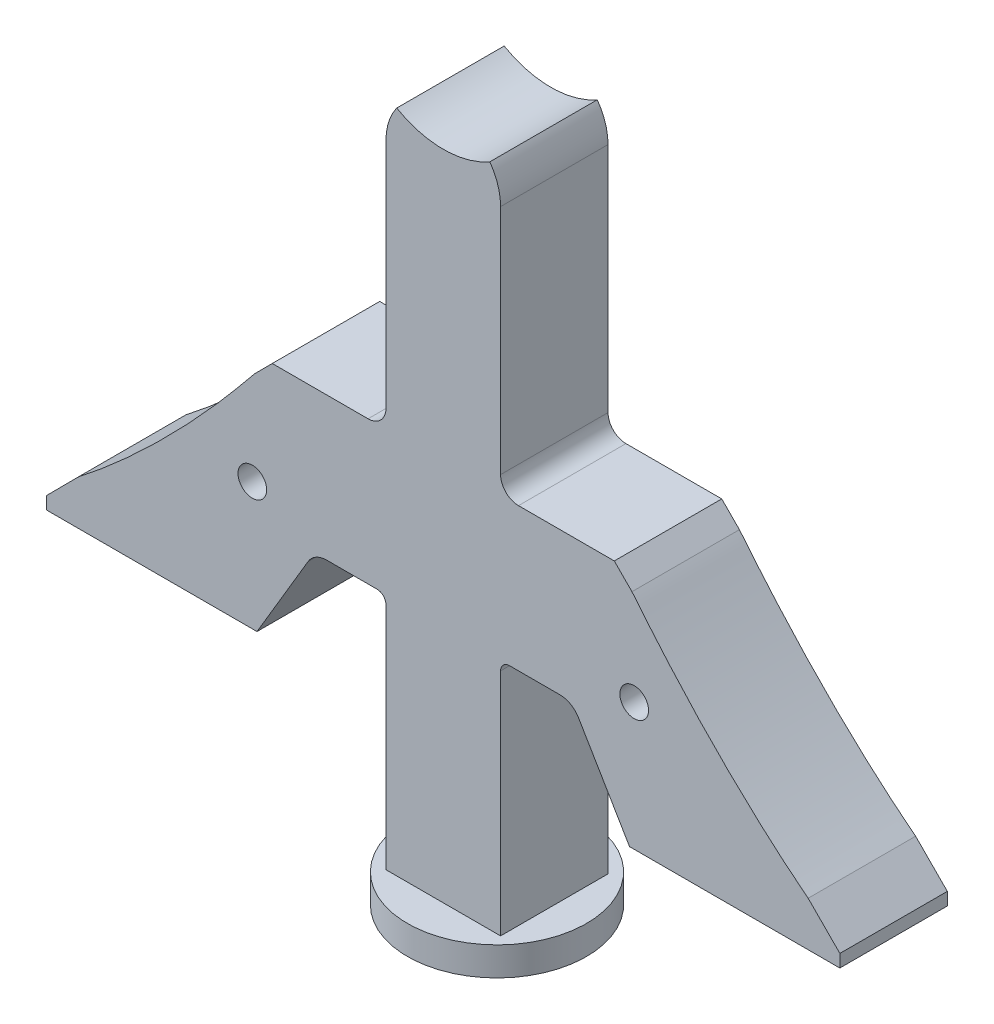
SolidWorks part; units mm, degrees
ref_plane "Front Plane" through (0, 0, 0) normal (0, 0, 1) x (1, 0, 0)
ref_plane "Top Plane" through (0, 0, 0) normal (0, 1, 0) x (1, 0, 0)
ref_plane "Right Plane" through (0, 0, 0) normal (1, 0, 0) x (0, 0, -1)
sketch "Sketch1" plane through (0, 0, 0) normal (0, 0, 1) x (1, 0, 0)
  line L0 (-15, 37.0303) -> (-15, -127.658)
  line L1 (15, 37.0303) -> (15, -127.658)
  line L2 (-15, -127.658) -> (15, -127.658)
  arc A3 (15, 37.0303) -> (-15, 37.0303) centre (0, 37.0303) ccw
extrude "Boss-Extrude1" add sketch "Sketch1" along normal blind 10
sketch "Sketch2" plane through (0, 0, 0) normal (0, 0, -1) x (-1, 0, 0)
  line L25 (0, -15) -> (30.09, -15)
  line L29 (139.2471, -124.8835) -> (-139.2471, -124.8835)
  line L30 (0, 159.5195) -> (0, -140.4805) construction
  line L31 (0, -15) -> (-30.09, -15)
  line L32 (30.09, -15) -> (139.2471, -124.8835)
  line L34 (-30.09, -15) -> (-139.2471, -124.8835)
  dimension "D1" = 45.19
  dimension "D2" = 45.19
  dimension "D3" = 30.09
  dimension "D4" = 30.09
extrude "Boss-Extrude2" add sketch "Sketch2" against normal blind 10
sketch "Sketch72" plane through (0, 0, 10) normal (0, 0, 1) x (1, 0, 0)
  circle A0 centre (0, 37.0303) radius 5
extrude "Cut-Extrude2" cut sketch "Sketch72" against normal blind 10
sketch "Sketch75" plane through (0, 0, 10) normal (0, 0, 1) x (1, 0, 0)
  line L2 (-101.3658, -86.7501) -> (-101.3003, -86.8152)
sketch "Sketch76" plane through (0, 0, 10) normal (0, 0, 1) x (1, 0, 0)
  line L2 (-100.6847, -86.0644) -> (-100.5316, -86.2165)
sketch "Sketch77" plane through (0, 0, 10) normal (0, 0, 1) x (1, 0, 0)
  line L2 (-99.9976, -85.3728) -> (-99.7607, -85.6082)
sketch "Sketch78" plane through (0, 0, 10) normal (0, 0, 1) x (1, 0, 0)
  circle A0 centre (-65.1228, -29.2131) radius 15
sketch "Sketch79" plane through (0, 0, 10) normal (0, 0, 1) x (1, 0, 0)
  circle A0 centre (-63.7391, -27.6067) radius 15
sketch "Sketch80" plane through (0, 0, 10) normal (0, 0, 1) x (1, 0, 0)
  line L2 (-99.3047, -84.6753) -> (-98.9873, -84.9906)
sketch "Sketch81" plane through (0, 0, 10) normal (0, 0, 1) x (1, 0, 0)
  line L2 (-98.6059, -83.9719) -> (-98.2113, -84.3638)
sketch "Sketch82" plane through (0, 0, 10) normal (0, 0, 1) x (1, 0, 0)
  line L2 (-97.9012, -83.2624) -> (-97.4325, -83.728)
sketch "Sketch83" plane through (0, 0, 10) normal (0, 0, 1) x (1, 0, 0)
  line L2 (-97.1906, -82.5471) -> (-96.6508, -83.0833)
sketch "Sketch84" plane through (0, 0, 10) normal (0, 0, 1) x (1, 0, 0)
  line L2 (-96.474, -81.8257) -> (-95.866, -82.4297)
sketch "Sketch85" plane through (0, 0, 10) normal (0, 0, 1) x (1, 0, 0)
  line L2 (-95.7514, -81.0984) -> (-95.078, -81.7673)
sketch "Sketch86" plane through (0, 0, 10) normal (0, 0, 1) x (1, 0, 0)
  line L2 (-95.0229, -80.365) -> (-94.2869, -81.0962)
sketch "Sketch88" plane through (0, 0, 10) normal (0, 0, 1) x (1, 0, 0)
  line L2 (-94.2885, -79.6257) -> (-93.4926, -80.4163)
sketch "Sketch89" plane through (0, 0, 10) normal (0, 0, 1) x (1, 0, 0)
  line L2 (-92.8017, -78.129) -> (-91.8942, -79.0305)
sketch "Sketch90" plane through (0, 0, 10) normal (0, 0, 1) x (1, 0, 0)
  line L1 (-93.5481, -78.8804) -> (-92.695, -79.7278)
sketch "Sketch91" plane through (0, 0, 10) normal (0, 0, 1) x (1, 0, 0)
  line L2 (-92.0494, -77.3717) -> (-91.0901, -78.3246)
sketch "Sketch92" plane through (0, 0, 10) normal (0, 0, 1) x (1, 0, 0)
  line L2 (-91.2911, -76.6083) -> (-90.2828, -77.61)
sketch "Sketch94" plane through (0, 0, 10) normal (0, 0, 1) x (1, 0, 0)
  line L2 (-89.7566, -75.0637) -> (-88.6584, -76.1546)
sketch "Sketch95" plane through (0, 0, 10) normal (0, 0, 1) x (1, 0, 0)
  line L2 (-90.5268, -75.839) -> (-89.4722, -76.8866)
sketch "Sketch96" plane through (0, 0, 10) normal (0, 0, 1) x (1, 0, 0)
  line L2 (-88.9805, -74.2823) -> (-87.8414, -75.4138)
sketch "Sketch97" plane through (0, 0, 10) normal (0, 0, 1) x (1, 0, 0)
  line L2 (-88.1983, -73.495) -> (-87.0213, -74.6643)
sketch "Sketch98" plane through (0, 0, 10) normal (0, 0, 1) x (1, 0, 0)
  line L2 (-87.4103, -72.7017) -> (-86.198, -73.906)
sketch "Sketch99" plane through (0, 0, 10) normal (0, 0, 1) x (1, 0, 0)
  line L2 (-86.6163, -71.9024) -> (-85.3716, -73.1388)
sketch "Sketch100" plane through (0, 0, 10) normal (0, 0, 1) x (1, 0, 0)
  line L2 (-85.8163, -71.0971) -> (-84.5422, -72.3629)
sketch "Sketch101" plane through (0, 0, 10) normal (0, 0, 1) x (1, 0, 0)
  line L2 (-85.0104, -70.2859) -> (-83.7097, -71.578)
sketch "Sketch102" plane through (0, 0, 10) normal (0, 0, 1) x (1, 0, 0)
  line L2 (-84.1986, -69.4686) -> (-82.8742, -70.7842)
sketch "Sketch103" plane through (0, 0, 10) normal (0, 0, 1) x (1, 0, 0)
  line L2 (-82.5572, -67.8163) -> (-81.1946, -69.1699)
sketch "Sketch104" plane through (0, 0, 10) normal (0, 0, 1) x (1, 0, 0)
  line L2 (-83.3808, -68.6454) -> (-82.0358, -69.9815)
sketch "Sketch105" plane through (0, 0, 10) normal (0, 0, 1) x (1, 0, 0)
  line L2 (-81.7276, -66.9812) -> (-80.3504, -68.3492)
sketch "Sketch106" plane through (0, 0, 10) normal (0, 0, 1) x (1, 0, 0)
  line L2 (-80.892, -66.1401) -> (-79.5035, -67.5194)
sketch "Sketch107" plane through (0, 0, 10) normal (0, 0, 1) x (1, 0, 0)
  line L2 (-80.0506, -65.2931) -> (-78.6539, -66.6806)
sketch "Sketch108" plane through (0, 0, 0) normal (0, 0, 1) x (1, 0, 0)
  line L2 (-79.2033, -64.4401) -> (-77.8016, -65.8326)
sketch "Sketch109" plane through (0, 0, 0) normal (0, 0, 1) x (1, 0, 0)
  line L2 (-78.3501, -63.5812) -> (-76.9466, -64.9754)
sketch "Sketch110" plane through (0, 0, 10) normal (0, 0, 1) x (1, 0, 0)
  line L2 (-77.4909, -62.7164) -> (-76.0891, -64.109)
sketch "Sketch111" plane through (0, 0, 10) normal (0, 0, 1) x (1, 0, 0)
  line L2 (-75.7551, -60.9689) -> (-74.3666, -62.3482)
sketch "Sketch112" plane through (0, 0, 10) normal (0, 0, 1) x (1, 0, 0)
  line L1 (-76.6259, -61.8456) -> (-75.2291, -63.2333)
sketch "Sketch113" plane through (0, 0, 10) normal (0, 0, 1) x (1, 0, 0)
  line L2 (-74.8783, -60.0863) -> (-73.5017, -61.4539)
sketch "Sketch115" plane through (0, 0, 10) normal (0, 0, 1) x (1, 0, 0)
  line L2 (-73.9957, -59.1978) -> (-72.6344, -60.5501)
sketch "Sketch116" plane through (0, 0, 10) normal (0, 0, 1) x (1, 0, 0)
  line L2 (-73.1072, -58.3034) -> (-71.7649, -59.6368)
sketch "Sketch117" plane through (0, 0, 10) normal (0, 0, 1) x (1, 0, 0)
  line L2 (-72.2128, -57.4031) -> (-70.8932, -58.714)
sketch "Sketch118" plane through (0, 0, 10) normal (0, 0, 1) x (1, 0, 0)
  line L2 (-71.3126, -56.4969) -> (-70.0193, -57.7817)
sketch "Sketch119" plane through (0, 0, 10) normal (0, 0, 1) x (1, 0, 0)
  line L2 (-70.4066, -55.5848) -> (-69.1433, -56.8397)
sketch "Sketch120" plane through (0, 0, 10) normal (0, 0, 1) x (1, 0, 0)
  line L2 (-69.4947, -54.6669) -> (-68.2654, -55.8881)
sketch "Sketch121" plane through (0, 0, 10) normal (0, 0, 1) x (1, 0, 0)
  line L2 (-68.577, -53.7431) -> (-67.3854, -54.9268)
sketch "Sketch122" plane through (0, 0, 10) normal (0, 0, 1) x (1, 0, 0)
  line L2 (-67.6534, -52.8134) -> (-66.5036, -53.9556)
sketch "Sketch123" plane through (0, 0, 10) normal (0, 0, 1) x (1, 0, 0)
  line L2 (-66.7241, -51.8778) -> (-65.6199, -52.9747)
sketch "Sketch124" plane through (0, 0, 10) normal (0, 0, 1) x (1, 0, 0)
  line L2 (-65.7889, -50.9365) -> (-64.7345, -51.9839)
sketch "Sketch125" plane through (0, 0, 10) normal (0, 0, 1) x (1, 0, 0)
  line L2 (-64.8479, -49.9892) -> (-63.8474, -50.9831)
sketch "Sketch126" plane through (0, 0, 10) normal (0, 0, 1) x (1, 0, 0)
  line L2 (-63.9012, -49.0361) -> (-62.9587, -49.9724)
sketch "Sketch127" plane through (0, 0, 10) normal (0, 0, 1) x (1, 0, 0)
  line L2 (-62.9486, -48.0772) -> (-62.0684, -48.9516)
sketch "Sketch128" plane through (0, 0, 10) normal (0, 0, 1) x (1, 0, 0)
  line L2 (-61.9903, -47.1125) -> (-61.1767, -47.9207)
sketch "Sketch129" plane through (0, 0, 10) normal (0, 0, 1) x (1, 0, 0)
  line L2 (-61.0261, -46.142) -> (-60.2836, -46.8796)
sketch "Sketch130" plane through (0, 0, 10) normal (0, 0, 1) x (1, 0, 0)
  line L2 (-60.0562, -45.1657) -> (-59.3892, -45.8283)
sketch "Sketch131" plane through (0, 0, 10) normal (0, 0, 1) x (1, 0, 0)
  line L2 (-59.0806, -44.1835) -> (-58.4935, -44.7668)
sketch "Sketch132" plane through (0, 0, 10) normal (0, 0, 1) x (1, 0, 0)
  line L2 (-58.0992, -43.1956) -> (-57.5966, -43.6949)
sketch "Sketch133" plane through (0, 0, 10) normal (0, 0, 1) x (1, 0, 0)
  line L2 (-57.1121, -42.2019) -> (-56.6986, -42.6126)
sketch "Sketch134" plane through (0, 0, 10) normal (0, 0, 1) x (1, 0, 0)
  line L2 (-56.1192, -41.2024) -> (-55.7997, -41.5198)
sketch "Sketch135" plane through (0, 0, 10) normal (0, 0, 1) x (1, 0, 0)
  line L2 (-55.1206, -40.1971) -> (-54.8997, -40.4165)
sketch "Sketch136" plane through (0, 0, 10) normal (0, 0, 1) x (1, 0, 0)
  line L2 (-54.1162, -39.1861) -> (-53.999, -39.3026)
sketch "Sketch137" plane through (0, 0, 10) normal (0, 0, 1) x (1, 0, 0)
  line L0 (-101.3003, -86.8152) -> (-100.5316, -86.2165)
  line L1 (-100.5316, -86.2165) -> (-99.7607, -85.6082)
  line L2 (-99.7607, -85.6082) -> (-98.9873, -84.9906)
  line L3 (-98.9873, -84.9906) -> (-98.2113, -84.3638)
  line L4 (-98.2113, -84.3638) -> (-97.4325, -83.728)
  line L5 (-97.4325, -83.728) -> (-96.6508, -83.0833)
  line L6 (-96.6508, -83.0833) -> (-95.866, -82.4297)
  line L7 (-95.866, -82.4297) -> (-95.078, -81.7673)
  line L8 (-95.078, -81.7673) -> (-94.2869, -81.0962)
  line L9 (-94.2869, -81.0962) -> (-93.4926, -80.4163)
  line L10 (-93.4926, -80.4163) -> (-92.695, -79.7278)
  line L11 (-92.695, -79.7278) -> (-91.8942, -79.0305)
  line L12 (-91.8942, -79.0305) -> (-91.0901, -78.3246)
  line L13 (-91.0901, -78.3246) -> (-90.2828, -77.61)
  line L14 (-90.2828, -77.61) -> (-89.4722, -76.8866)
  line L15 (-89.4722, -76.8866) -> (-88.6584, -76.1546)
  line L16 (-88.6584, -76.1546) -> (-87.8414, -75.4138)
  line L17 (-87.8414, -75.4138) -> (-87.0213, -74.6643)
  line L18 (-87.0213, -74.6643) -> (-86.198, -73.906)
  line L19 (-86.198, -73.906) -> (-85.3716, -73.1388)
  line L20 (-85.3716, -73.1388) -> (-84.5422, -72.3629)
  line L21 (-84.5422, -72.3629) -> (-83.7097, -71.578)
  line L22 (-83.7097, -71.578) -> (-82.8742, -70.7842)
  line L23 (-82.8742, -70.7842) -> (-82.0358, -69.9815)
  line L24 (-82.0358, -69.9815) -> (-81.1946, -69.1699)
  line L25 (-81.1946, -69.1699) -> (-80.3504, -68.3492)
  line L26 (-80.3504, -68.3492) -> (-79.5035, -67.5194)
  line L27 (-79.5035, -67.5194) -> (-78.6539, -66.6806)
  line L28 (-78.6539, -66.6806) -> (-77.8016, -65.8326)
  line L29 (-77.8016, -65.8326) -> (-76.9466, -64.9754)
  line L30 (-76.9466, -64.9754) -> (-76.0891, -64.109)
  line L31 (-76.0891, -64.109) -> (-75.2291, -63.2333)
  line L32 (-75.2291, -63.2333) -> (-74.3666, -62.3482)
  line L33 (-74.3666, -62.3482) -> (-73.5017, -61.4539)
  line L34 (-73.5017, -61.4539) -> (-72.6344, -60.5501)
  line L35 (-72.6344, -60.5501) -> (-71.7649, -59.6368)
  line L36 (-71.7649, -59.6368) -> (-70.8932, -58.714)
  line L37 (-70.8932, -58.714) -> (-70.0193, -57.7817)
  line L38 (-70.0193, -57.7817) -> (-69.1433, -56.8397)
  line L39 (-69.1433, -56.8397) -> (-68.2654, -55.8881)
  line L40 (-68.2654, -55.8881) -> (-67.3854, -54.9268)
  line L41 (-67.3854, -54.9268) -> (-66.5036, -53.9556)
  line L42 (-66.5036, -53.9556) -> (-65.6199, -52.9747)
  line L43 (-65.6199, -52.9747) -> (-64.7345, -51.9839)
  line L44 (-64.7345, -51.9839) -> (-63.8474, -50.9831)
  line L45 (-63.8474, -50.9831) -> (-62.9587, -49.9724)
  line L46 (-62.9587, -49.9724) -> (-62.0684, -48.9516)
  line L47 (-62.0684, -48.9516) -> (-61.1767, -47.9207)
  line L48 (-61.1767, -47.9207) -> (-60.2836, -46.8796)
  line L49 (-60.2836, -46.8796) -> (-59.3892, -45.8283)
  line L50 (-59.3892, -45.8283) -> (-58.4935, -44.7668)
  line L51 (-58.4935, -44.7668) -> (-57.5966, -43.6949)
  line L52 (-57.5966, -43.6949) -> (-56.6986, -42.6126)
  line L53 (-56.6986, -42.6126) -> (-55.7997, -41.5198)
  line L54 (-55.7997, -41.5198) -> (-54.8997, -40.4165)
  line L55 (-54.8997, -40.4165) -> (-53.999, -39.3026)
sketch "Sketch162" plane through (0, 0, 10) normal (0, 0, 1) x (1, 0, 0)
  line L0 (-101.3519, -86.7361) -> (-100.0146, -88.0645)
  line L1 (-102.628, -87.9737) -> (-101.2862, -89.6675)
  line L2 (-101.8673, -87.2549) -> (-101.8304, -87.2953)
  line L3 (-101.8304, -87.2953) -> (-101.4956, -87.6621)
  line L4 (-106.6713, -92.0909) -> (-96.0905, -81.4397)
  line L5 (-139.2471, -124.8835) -> (-30.09, -15) construction
sketch "Sketch140" plane through (0, 0, 10) normal (0, 0, 1) x (1, 0, 0)
  circle A0 centre (0, 37.0303) radius 15
sketch "Sketch144" plane through (0, 0, 10) normal (0, 0, 1) x (1, 0, 0)
  line L0 (-13, 37.0303) -> (-13, -15)
  line L1 (13, 37.0303) -> (13, -15)
  line L2 (23, 37.0303) -> (23, -15)
  line L4 (-23, 37.0303) -> (-23, -15)
  line L5 (-13, -15) -> (-23, -15)
  line L6 (13, -15) -> (23, -15)
  arc A0 (13, 37.0303) -> (-13, 37.0303) centre (0, 37.0303) ccw
  arc A1 (23, 37.0303) -> (-23, 37.0303) centre (0, 37.0303) ccw
  dimension "D1" = 10
extrude "Cut-Extrude4" cut sketch "Sketch144" against normal blind 19 and the other way blind 14
sketch "Sketch145" plane through (0, 0, 0) normal (0, 0, -1) x (-1, 0, 0)
  line L15 (30.09, -15) -> (13, -15)
  line L16 (13, -15) -> (13, 37.0303)
  line L17 (-13, 37.0303) -> (-13, -15)
  line L18 (-13, -15) -> (-30.09, -15)
  line L19 (-30.09, -15) -> (-139.2471, -124.8835)
  line L22 (-139.2471, -124.8835) -> (-15, -124.8835)
  line L23 (-15, -124.8835) -> (-15, -127.658)
  line L24 (-15, -127.658) -> (15, -127.658)
  line L25 (15, -127.658) -> (15, -124.8835)
  line L26 (15, -124.8835) -> (139.2471, -124.8835)
  line L27 (139.2471, -124.8835) -> (30.09, -15)
  line L30 (30.09, -15) -> (13, -15)
  line L31 (13, -15) -> (13, 37.0303)
  line L32 (-13, 37.0303) -> (-13, -15)
  line L33 (-13, -15) -> (-30.09, -15)
  line L34 (-30.09, -15) -> (-139.2471, -124.8835)
  line L37 (-139.2471, -124.8835) -> (-15, -124.8835)
  line L38 (-15, -124.8835) -> (-15, -127.658)
  line L39 (-15, -127.658) -> (15, -127.658)
  line L40 (15, -127.658) -> (15, -124.8835)
  line L41 (15, -124.8835) -> (139.2471, -124.8835)
  line L42 (139.2471, -124.8835) -> (30.09, -15)
  arc A1 (13, 37.0303) -> (-13, 37.0303) centre (0, 37.0303) ccw
  arc A2 (13, 37.0303) -> (-13, 37.0303) centre (0, 37.0303) ccw
  dimension "D1" = 0
extrude "Boss-Extrude3" add sketch "Sketch145" along normal blind 20
sketch "Sketch146" plane through (0, 0, 0) normal (0, 0, 1) x (1, 0, 0)
  circle A1 centre (0, 37.0303) radius 5
extrude "Cut-Extrude5" cut sketch "Sketch146" against normal blind 48 and the other way blind 19
sketch "Sketch147" plane through (0, 0, 0) normal (1, 0, 0) x (0, 0, -1)
  line L1 (-2.5, 50.0303) -> (-2.5, 20.0303)
  line L8 (-2.5, 50.0303) -> (5, 50.0303)
  line L10 (12.5, 50.0303) -> (12.5, 20.0303)
  line L18 (-2.5, 20.0303) -> (12.5, 20.0303)
  line L19 (20, 50.0303) -> (-10, 50.0303) construction
  line L20 (5, 50.0303) -> (12.5, 50.0303)
  dimension "D1" = 30
extrude "Cut-Extrude6" cut sketch "Sketch147" against normal blind 19 and the other way blind 19
sketch "Sketch150" plane through (0, 0, 10) normal (0, 0, 1) x (1, 0, 0)
  line L0 (-139.2471, -124.8835) -> (-114.2471, -124.8835)
  line L1 (-15, -124.8835) -> (-139.2471, -124.8835) construction
  line L2 (-114.2471, -124.8835) -> (-114.2471, -93.8389)
  line L3 (-114.2471, -93.8389) -> (-155.6043, -93.8389)
  line L4 (-155.6043, -93.8389) -> (-139.2471, -124.8835)
  line L5 (139.2471, -124.8835) -> (114.2471, -124.8835)
  line L6 (139.2471, -124.8835) -> (15, -124.8835) construction
  line L7 (114.2471, -124.8835) -> (114.2471, -93.8389)
  line L8 (114.2471, -93.8389) -> (144.7788, -93.8389)
  line L9 (144.7788, -93.8389) -> (139.2471, -124.8835)
extrude "Cut-Extrude7" cut sketch "Sketch150" against normal blind 60
sketch "Sketch151" plane through (0, 0, 10) normal (0, 0, 1) x (1, 0, 0)
  circle A2 centre (-53.3051, -64.1314) radius 4
sketch "Sketch153" plane through (0, 0, 10) normal (0, 0, 1) x (1, 0, 0)
  circle A1 centre (53.3051, -64.1314) radius 4
sketch "Sketch154" plane through (0, 0, -20) normal (0, 0, -1) x (-1, 0, 0)
  line L0 (-13, 37.0303) -> (-13, -127.658)
  line L1 (-15, -127.658) -> (15, -127.658) construction
  line L2 (13, 37.0303) -> (13, -127.658)
  line L3 (13, -127.658) -> (-13, -127.658)
  arc A0 (13, 37.0303) -> (-13, 37.0303) centre (0, 37.0303) ccw construction
  arc A1 (13, 37.0303) -> (-13, 37.0303) centre (0, 37.0303) ccw
sketch "Sketch155" plane through (0, 0, -20) normal (0, 0, -1) x (-1, 0, 0)
  line L0 (-114.2471, -99.7171) -> (114.2471, -99.7171)
  line L1 (114.2471, -99.7171) -> (132.9981, -127.2807)
  line L2 (132.9981, -127.2807) -> (-4.839, -174.8107)
  line L3 (-4.839, -174.8107) -> (-128.9451, -139.6913)
  line L4 (-128.9451, -139.6913) -> (-114.2471, -99.7171)
extrude "Cut-Extrude8" cut sketch "Sketch155" against normal blind 72
sketch "Sketch156" plane through (0, 0, -20) normal (0, 0, -1) x (-1, 0, 0)
  line L0 (-13, 20.0896) -> (-13, -102.7368)
  line L1 (-13, 37.0303) -> (-13, -15) construction
  line L2 (13, 22.765) -> (13, -108.8173)
  line L3 (13, -15) -> (13, 37.0303) construction
sketch "Sketch161" plane through (0, 0, -20) normal (0, 0, -1) x (-1, 0, 0)
  line L0 (0, 27.3777) -> (0, -17.3471)
sketch "Sketch164" plane through (0, 0, 10) normal (0, 0, 1) x (1, 0, 0)
  circle A0 centre (0, 37.0303) radius 15
sketch "Sketch165" plane through (0, 0, 10) normal (0, 0, 1) x (1, 0, 0)
  line L1 (-100.4199, -86.2739) -> (-99.4234, -87.2638)
sketch "Sketch166" plane through (0, 0, 10) normal (0, 0, 1) x (1, 0, 0)
  line L1 (-99.7607, -85.6082) -> (-98.894, -86.4688)
sketch "Sketch167" plane through (0, 0, 10) normal (0, 0, 1) x (1, 0, 0)
  line L0 (-112.3258, -76.5395) -> (-101.6841, -87.1108)
sketch "Sketch168" plane through (0, 0, 10) normal (0, 0, 1) x (1, 0, 0)
  line L0 (-114.2471, -99.7171) -> (-30.09, -15) construction
  line L1 (-102.628, -87.9737) -> (-98.2113, -23.8388)
  line L2 (-98.2113, -23.8388) -> (-52.6767, -37.737)
  circle A0 centre (-63.7391, -27.6067) radius 15 construction
  spline S0 degree 3 poles (-52.6767, -37.737) (-53.4483, -38.6049) (-54.758, -40.2555) (-56.3933, -42.2454) (-57.5939, -43.6933) (-58.4909, -44.7652) (-59.3866, -45.8268) (-60.281, -46.878) (-61.1741, -47.9191) (-62.0659, -48.95) (-62.9561, -49.9708) (-63.8448, -50.9816) (-64.7319, -51.9823) (-65.6174, -52.9732) (-66.501, -53.9541) (-67.3829, -54.9252) (-68.2628, -55.8866) (-69.1408, -56.8382) (-70.0168, -57.7802) (-70.8907, -58.7125) (-71.7624, -59.6353) (-72.6319, -60.5486) (-73.4991, -61.4524) (-74.364, -62.3468) (-75.2265, -63.2318) (-76.0866, -64.1075) (-76.9441, -64.9739) (-77.7991, -65.8311) (-78.6514, -66.6791) (-79.501, -67.518) (-80.3479, -68.3478) (-81.1921, -69.1685) (-82.0333, -69.9802) (-82.8717, -70.7829) (-83.7072, -71.5766) (-84.5396, -72.3615) (-85.3691, -73.1375) (-86.1955, -73.9046) (-87.0188, -74.663) (-87.8389, -75.4125) (-88.6559, -76.1533) (-89.4697, -76.8854) (-90.2803, -77.6087) (-91.0876, -78.3233) (-91.8917, -79.0293) (-92.6925, -79.7265) (-93.4901, -80.4151) (-94.2844, -81.095) (-95.0755, -81.7662) (-95.8634, -82.4286) (-96.6482, -83.0822) (-97.43, -83.727) (-98.2088, -84.3629) (-98.9847, -84.9897) (-99.758, -85.6074) (-100.5291, -86.2155) (-101.1703, -86.7164) (-101.8954, -87.2708) (-102.3524, -87.6414) (-102.628, -87.9737) knots 0 0 0 0 0.049043 0.089028 0.108836 0.128522 0.148086 0.167528 0.186848 0.206047 0.225125 0.244082 0.262919 0.281636 0.300232 0.318708 0.337065 0.355302 0.373421 0.39142 0.4093 0.427061 0.444704 0.462229 0.479635 0.496923 0.514094 0.531146 0.548081 0.564899 0.581599 0.598182 0.614648 0.630996 0.647228 0.663343 0.679342 0.695224 0.71099 0.72664 0.742173 0.757591 0.772893 0.788079 0.803151 0.818107 0.832948 0.847675 0.862288 0.876786 0.891172 0.905445 0.919606 0.933656 0.947596 0.961428 0.975152 0.981975 1 1 1 1
extrude "Cut-Extrude9" cut sketch "Sketch168" against normal blind 88
mirror "Mirror1" about plane through (0, 0, 0) normal (1, 0, 0) of "Cut-Extrude9"
sketch "Sketch169" plane through (0, 0, 10) normal (0, 0, 1) x (1, 0, 0)
  line L8 (-16, -15) -> (-13, -15)
  line L10 (-30.09, -15) -> (-13, -15) construction
  line L11 (13, -15) -> (30.09, -15) construction
  line L12 (0, -15) -> (0, 37.0303) construction
  line L13 (-16, -15) -> (-16, 37.0303)
  line L14 (-16, 37.0303) -> (0, 37.0303) construction
  line L15 (16, -15) -> (16, 37.0303)
  line L16 (-16, 37.0303) -> (-10.5625, 44.6087)
  line L17 (16, 37.0303) -> (10.5625, 44.6087)
  line L18 (13, -15) -> (13, 37.0303) construction
  line L19 (-13, 37.0303) -> (-13, -15) construction
  line L20 (13, -15) -> (13, 37.0303)
  line L21 (-13, 37.0303) -> (-13, -15)
  line L22 (13, -15) -> (16, -15)
  circle A5 centre (0, 37.0303) radius 5 construction
  arc A6 (13, 37.0303) -> (-13, 37.0303) centre (0, 37.0303) ccw construction
  arc A7 (13, 37.0303) -> (10.5625, 44.6087) centre (0, 37.0303) ccw
  arc A8 (-10.5625, 44.6087) -> (-13, 37.0303) centre (0, 37.0303) ccw
  dimension "D1" = 32
extrude "Boss-Extrude6" add sketch "Sketch169" against normal up to surface (7.5 mm away) up to face at (0, 31.7803, 2.5)
sketch "Sketch170" plane through (0, 0, 10) normal (0, 0, 1) x (1, 0, 0)
  line L0 (-63.8875, -32.7712) -> (-27.1884, -2.7408)
  line L2 (-27.1884, -2.7408) -> (-16, -2.7408)
  line L4 (-16, -2.7408) -> (-16, -15)
  line L5 (-63.8875, -32.7712) -> (-16, -32.7712)
  line L7 (-16, -15) -> (-16, -32.7712)
  line L8 (16, -15) -> (16, -32.7712)
  line L9 (63.8875, -32.7712) -> (16, -32.7712)
  line L10 (16, -2.7408) -> (16, -15)
  line L11 (27.1884, -2.7408) -> (16, -2.7408)
  line L12 (63.8875, -32.7712) -> (27.1884, -2.7408)
extrude "Cut-Extrude10" cut sketch "Sketch170" against normal blind 41 and the other way blind 19
sketch "Sketch171" plane through (0, 0, -20) normal (0, 0, -1) x (-1, 0, 0)
  line L9 (16, -15) -> (-16, -15)
  line L10 (-16, -15) -> (-16, 37.0303)
  line L11 (-16, 37.0303) -> (-10.5625, 44.6087)
  line L12 (16, -15) -> (16, 37.0303)
  line L13 (16, 37.0303) -> (10.5625, 44.6087)
  arc A0 (10.5625, 44.6087) -> (-10.5625, 44.6087) centre (0, 37.0303) ccw construction
  arc A1 (10.5625, 44.6087) -> (-10.5625, 44.6087) centre (0, 37.0303) ccw
  circle A2 centre (0, 37.0303) radius 5
extrude "Boss-Extrude7" add sketch "Sketch171" against normal up to surface (7.5 mm away) up to face at (0, 31.7803, -12.5)
sketch "Sketch172" plane through (0, 0, 2.5) normal (0, 0, -1) x (-1, 0, 0)
  line L0 (-13, 20.0303) -> (-16, 20.0303)
  line L2 (-16, 20.0303) -> (-16, -15)
  line L3 (-16, -15) -> (-13, -15)
  line L4 (-13, -15) -> (-13, 20.0303)
  line L5 (13, 20.0303) -> (16, 20.0303)
  line L7 (16, 20.0303) -> (16, -15)
  line L8 (16, -15) -> (13, -15)
  line L9 (13, -15) -> (13, 20.0303)
extrude "Boss-Extrude8" add sketch "Sketch172" along normal up to surface (15 mm away) up to face at (0, 14.876, -12.5)
sketch "Sketch173" plane through (0, 0, -20) normal (0, 0, -1) x (-1, 0, 0)
  line L1 (114.2471, -99.7171) -> (-114.2471, -99.7171) construction
  line L2 (-16, -299.7171) -> (16, -299.7171)
  line L3 (16, -99.7171) -> (16, -299.7171)
  line L4 (-16, -99.7171) -> (16, -99.7171)
  line L5 (-16, -99.7171) -> (-16, -299.7171)
extrude "Boss-Extrude9" add sketch "Sketch173" against normal up to surface (30 mm away)
chamfer "Chamfer1" distance 5 angle 45 2 edges at (114.2471, -99.7171, -5) (-114.2471, -99.7171, -5)
fillet "Fillet1" radius 5 2 edges at (16, -32.7712, -5) (-16, -32.7712, -5)
sketch "Sketch174" plane through (0, 0, 10) normal (0, 0, 1) x (1, 0, 0)
  line L0 (-16, -99.7171) -> (-16, -75.2171)
  line L1 (-18.5, -72.7171) -> (-32.5812, -72.7171)
  line L3 (-16, -99.7171) -> (-110.7116, -99.7171) construction
  line L4 (-37.7429, -75.6583) -> (-52, -99.7171)
  line L5 (-16, -99.7171) -> (-52, -99.7171)
  line L6 (16, -99.7171) -> (52, -99.7171)
  line L7 (37.7429, -75.6583) -> (52, -99.7171)
  line L8 (18.5, -72.7171) -> (32.5812, -72.7171)
  line L9 (16, -99.7171) -> (16, -75.2171)
  arc A3 (32.5812, -72.7171) -> (37.7429, -75.6583) centre (32.5812, -78.7171) cw
  arc A4 (-37.7429, -75.6583) -> (-32.5812, -72.7171) centre (-32.5812, -78.7171) cw
  arc A5 (-16, -75.2171) -> (-18.5, -72.7171) centre (-18.5, -75.2171) ccw
  arc A6 (16, -75.2171) -> (18.5, -72.7171) centre (18.5, -75.2171) cw
  point P8 (-16, -72.7171)
  point P19 (16, -72.7171)
  point P22 (-36, -72.7171)
  dimension "D3" = 2.5
  dimension "D4" = 2.5
  dimension "D5" = 6
  dimension "D1" = 36
  dimension "D2" = 20
extrude "Cut-Extrude11" cut sketch "Sketch174" against normal blind 30
sketch "Sketch175" plane through (0, 0, 10) normal (0, 0, 1) x (1, 0, 0)
  line L2 (-27, -139.3028) -> (20.7687, -139.3028)
  line L3 (20.7687, -139.3028) -> (20.7687, -324.4548)
  line L4 (20.7687, -324.4548) -> (-27, -324.4548)
  line L5 (-27, -324.4548) -> (-27, -139.3028)
extrude "Cut-Extrude12" cut sketch "Sketch175" against normal blind 55
extrude "Cut-Extrude14" cut sketch "Sketch151" against normal blind 15 contours A2
extrude "Cut-Extrude15" cut sketch "Sketch153" against normal blind 15 contours A1
chamfer "Chamfer3" distance 0.5 angle 45 12 edges at (16, 20.0303, -5) (-16, 20.0303, -5) (0, 50.0303, 2.5) (0, 20.0303, 2.5) (-5, 37.0303, 2.5) (0, 50.0303, -12.5) (16, 28.5303, 2.5) (13.2812, 40.8195, 2.5) (-13.2813, 40.8195, 2.5) (-16, 28.5303, 2.5) (-13.2813, 40.8195, -12.5) (13.2812, 40.8195, -12.5)
ref_plane "Plane1" through (0, 0, 8.5) normal (0, 0, 1) x (1, 0, 0)
ref_plane "Plane2" through (0, 0, -18.5) normal (0, 0, -1) x (-1, 0, 0)
sketch "Sketch177" plane through (0, 0, 10) normal (0, 0, 1) x (1, 0, 0)
  line L0 (16, -27.7712) -> (16, 37.0303) construction
  line L1 (-16, 37.0303) -> (-16, -27.7712) construction
  line L2 (-16, 37.0303) -> (-16, -27.7712)
  line L3 (16, -27.7712) -> (16, 37.0303)
  line L4 (-16, -27.7712) -> (16, -27.7712)
  arc A0 (16, 37.0303) -> (-16, 37.0303) centre (0, 37.0303) ccw
extrude "Boss-Extrude10" add sketch "Sketch177" against normal up to surface (30 mm away) up to face at (0, -56.0165, -20)
sketch "Sketch178" plane through (0, 0, 10) normal (0, 0, 1) x (1, 0, 0)
  line L0 (0, 0) -> (0, 68.8743) construction
  line L1 (0, 68.8743) -> (-13, 46.3576)
  line L2 (0, 68.8743) -> (13, 46.3576)
  arc A0 (-13, 46.3576) -> (13, 46.3576) centre (0, 68.8743) ccw
  arc A1 (16, 37.0303) -> (-16, 37.0303) centre (0, 37.0303) ccw construction
  dimension "D2" = 52
  dimension "D1" = 60
extrude "Cut-Extrude16" cut sketch "Sketch178" against normal through all
sketch "Sketch179" plane through (0, -139.3028, 0) normal (0, -1, 0) x (1, 0, 0)
  line L0 (0, 10) -> (0, -20) construction
  line L1 (16, 10) -> (-16, 10) construction
  line L2 (-16, -20) -> (16, -20) construction
  line L3 (-16, -5) -> (16, -5) construction
  line L4 (-16, -20) -> (-16, 10) construction
  line L5 (16, -20) -> (16, 10) construction
  circle A0 centre (0, -5) radius 25
  dimension "D1" = 50
extrude "Boss-Extrude11" add sketch "Sketch179" along normal blind 8
